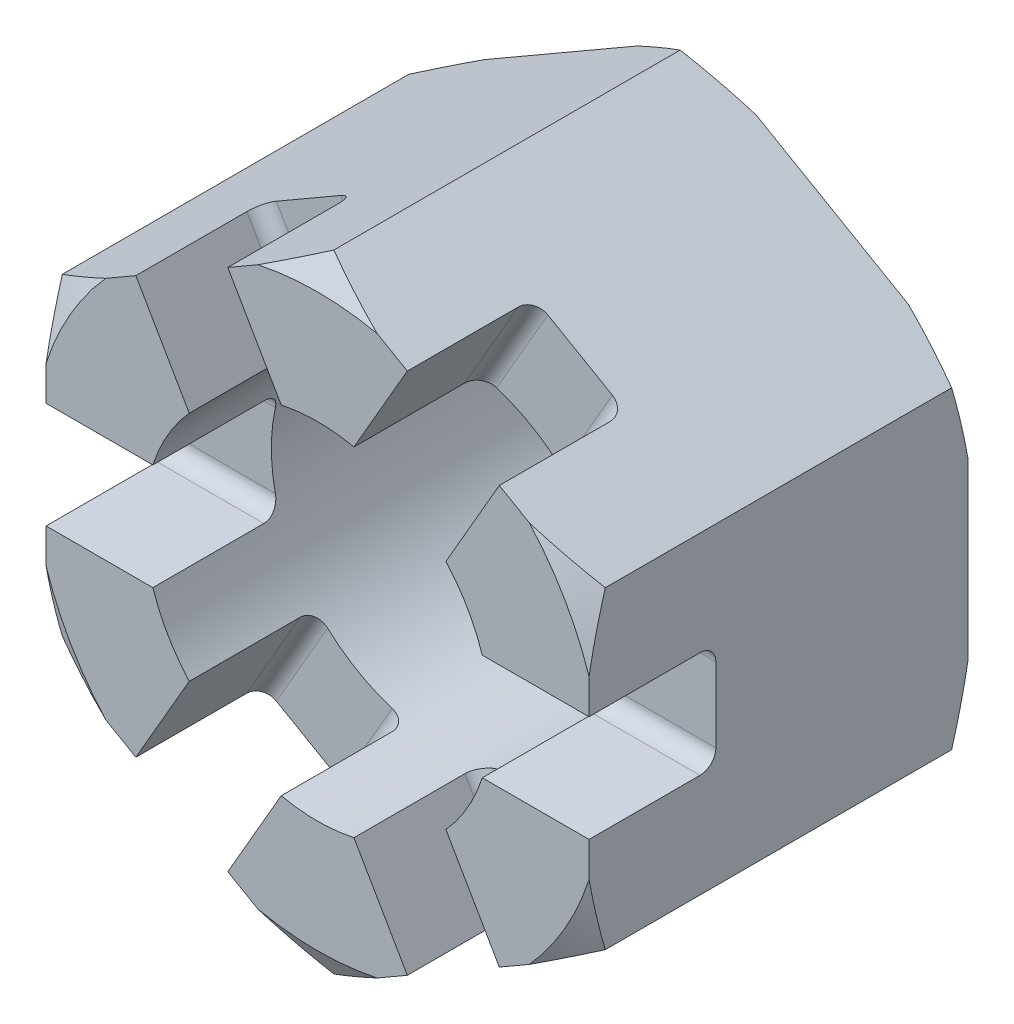
from build123d import *

# Parameters (mm, degrees)
SKETCH_1_R               = 10.9175
EXTRUDE_814_DEPTH        = 23.9
SKETCH_2_OUTSIDE_W       = 173.966
SKETCH_2_OUTSIDE_H       = 179.264
SKETCH_2_OUTSIDE_R       = 18
CUT_EXTRUDE_1_DEPTH      = 36.433721139
CUT_EXTRUDE_1_DRAFT      = -60
SKETCH_3_OUTSIDE_W       = 173.966
SKETCH_3_OUTSIDE_H       = 179.264
SKETCH_3_OUTSIDE_R       = 18
CUT_EXTRUDE_2_DEPTH      = 36.433721139
CUT_EXTRUDE_2_DRAFT      = -60
CUT_EXTRUDE_3_DEPTH      = 47.210523693
PATTERN_CIRCULAR_1_COUNT = 3
CHAMFER_1_SIZE           = 0.380357143


with BuildPart() as part:
    # 草图1 → Extrude 814 (new body)
    with BuildSketch(Plane.XY):
        Polygon((0, 19.775), (-17.12565236, 9.8875), (-17.12565236, -9.8875), (0, -19.775), (17.12565236, -9.8875), (17.12565236, 9.8875), align=None)
        with Locations(Location((0, 0, 0), (0, 0, 180))):
            Circle(SKETCH_1_R, mode=Mode.SUBTRACT)
    extrude(amount=EXTRUDE_814_DEPTH)


with BuildPart() as cut_extrude_1_tool:
    # 草图2 outside → 切除-拉伸1 (with draft: the straight prism first)
    with BuildSketch(Plane(origin=(0, 0, 0), x_dir=(-1, 0, 0), z_dir=(0, 0, -1))):
        Rectangle(SKETCH_2_OUTSIDE_W, SKETCH_2_OUTSIDE_H)
        Circle(SKETCH_2_OUTSIDE_R, mode=Mode.SUBTRACT)
    extrude(amount=-CUT_EXTRUDE_1_DEPTH)
    # 切除-拉伸1: the draft: its side faces are tilted about the plane it starts from
    cut_extrude_1_sides = [cut_extrude_1_tool.faces().sort_by_distance(p)[0] for p in [
        (0, -89.632, 18.216860569),
        (-86.983, 0, 18.216860569),
        (0, 89.632, 18.216860569),
        (86.983, 0, 18.216860569),
        (18, 0, 18.216860569),
    ]]
    draft(cut_extrude_1_sides, Plane(origin=(0, 0, 0), x_dir=(-1, 0, 0), z_dir=(0, 0, -1)), CUT_EXTRUDE_1_DRAFT)


with BuildPart() as part_1:
    add(part.part)

    # 切除-拉伸1: cut by cut_extrude_1_tool
    add(cut_extrude_1_tool.part, mode=Mode.SUBTRACT)


with BuildPart() as cut_extrude_2_tool:
    # 草图3 outside → 切除-拉伸2 (with draft: the straight prism first)
    with BuildSketch(Plane.XY.offset(23.9)):
        Rectangle(SKETCH_3_OUTSIDE_W, SKETCH_3_OUTSIDE_H)
        Circle(SKETCH_3_OUTSIDE_R, mode=Mode.SUBTRACT)
    extrude(amount=-CUT_EXTRUDE_2_DEPTH)
    # 切除-拉伸2: the draft: its side faces are tilted about the plane it starts from
    cut_extrude_2_sides = [cut_extrude_2_tool.faces().sort_by_distance(p)[0] for p in [
        (0, -89.632, 5.683139431),
        (86.983, 0, 5.683139431),
        (0, 89.632, 5.683139431),
        (-86.983, 0, 5.683139431),
        (-18, 0, 5.683139431),
    ]]
    draft(cut_extrude_2_sides, Plane.XY.offset(23.9), CUT_EXTRUDE_2_DRAFT)


with BuildPart() as part_2:
    add(part_1.part)

    # 切除-拉伸2: cut by cut_extrude_2_tool
    add(cut_extrude_2_tool.part, mode=Mode.SUBTRACT)

    # 草图6 → 切除-拉伸3 (cut, through all)
    with BuildSketch(Plane(origin=(17.12565236, 0, 0), x_dir=(0, 0, -1), z_dir=(1, 0, 0))):
        with BuildLine():
            Line((-23.9, -3.35), (-23.9, 3.35))
            Line((-23.9, 3.35), (-16.9, 3.35))
            ThreePointArc((-16.9, 3.35), (-16.192893219, 3.057106781), (-15.9, 2.35))
            Line((-15.9, 2.35), (-15.9, -2.35))
            ThreePointArc((-15.9, -2.35), (-16.192893219, -3.057106781), (-16.9, -3.35))
            Line((-16.9, -3.35), (-23.9, -3.35))
        make_face()
    cut_extrude_3 = extrude(amount=-CUT_EXTRUDE_3_DEPTH, mode=Mode.SUBTRACT)

    # 阵列(圆周)1: 切除-拉伸3 ×3 about axis
    pattern_circular_1_axis = Axis((0, 0, 0), (0, 0, 1))
    for i in range(1, PATTERN_CIRCULAR_1_COUNT):
        add(cut_extrude_3.rotate(pattern_circular_1_axis, i * 360 / PATTERN_CIRCULAR_1_COUNT), mode=Mode.SUBTRACT)

    # 倒角1
    chamfer_1_edges = [part_2.edges().sort_by_distance(p)[0] for p in [
        (10.9175, 0, 0),
    ]]
    chamfer(chamfer_1_edges, length=CHAMFER_1_SIZE)


solid = part_2.part
